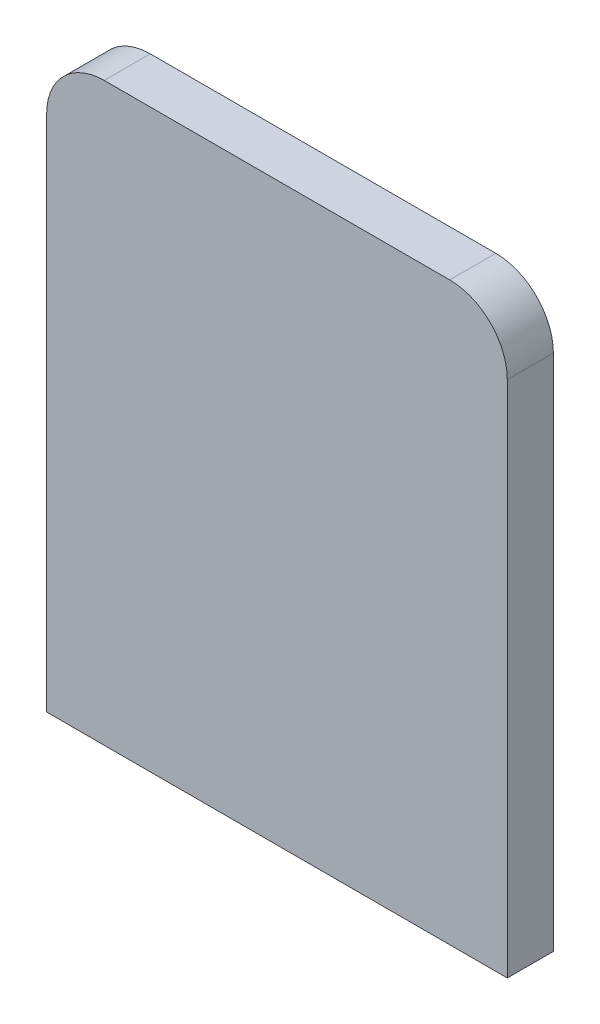
SolidWorks part; units mm, degrees
material "Plain carbon steel"
ref_plane "Front Plane" through (0, 0, 0) normal (0, 0, 1) x (1, 0, 0)
ref_plane "Top Plane" through (0, 0, 0) normal (0, 1, 0) x (1, 0, 0)
ref_plane "Right Plane" through (0, 0, 0) normal (1, 0, 0) x (0, 0, -1)
sketch "Sketch1" plane through (0, 0, 0) normal (0, 0, 1) x (1, 0, 0)
  line L1 (0, 0) -> (80, 0)
  line L2 (0, 0) -> (0, -100)
  line L3 (0, -100) -> (80, -100)
  line L4 (80, 0) -> (80, -100)
  line L5 (0, 0) -> (80, -100) construction
  line L6 (0, -100) -> (80, 0) construction
  point P4 (40, -50)
  dimension "D1" = 80
  dimension "D2" = 100
extrude "Boss-Extrude1" add sketch "Sketch1" along normal blind 8
fillet "Fillet1" radius 10 2 edges at (0, 0, 4) (80, 0, 4)
